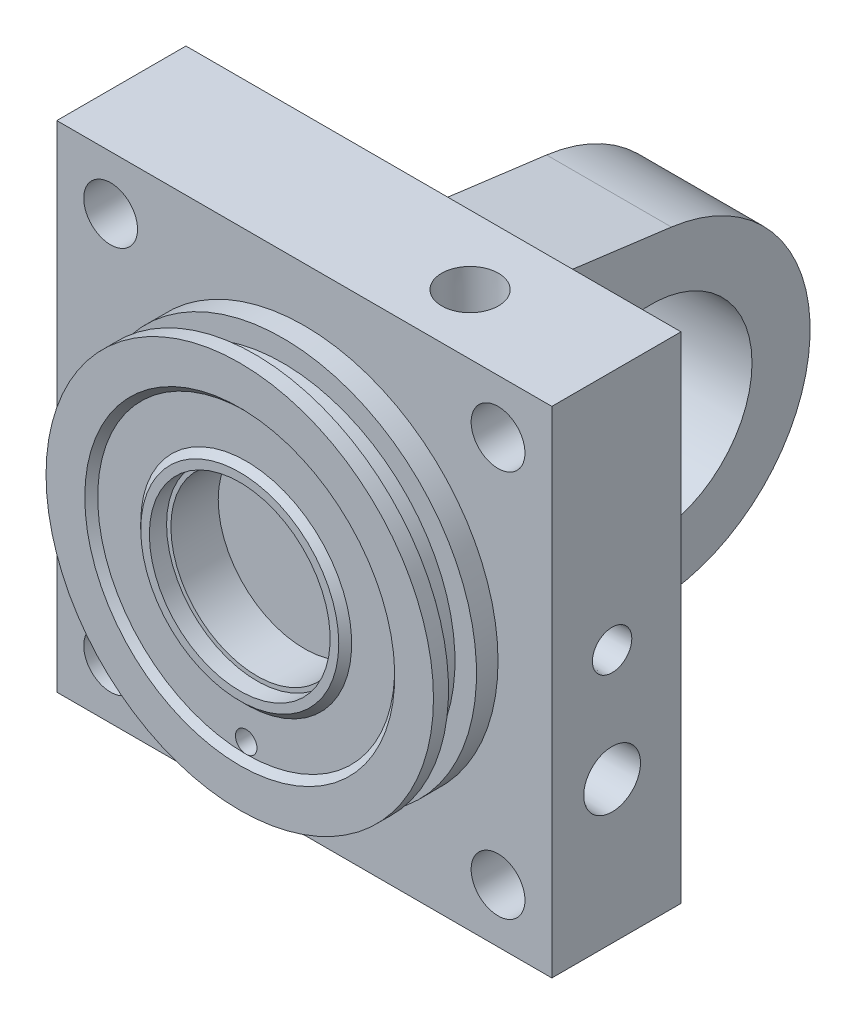
SolidWorks part; units mm, degrees
ref_plane "前视基准面" through (0, 0, 0) normal (0, 0, 1) x (1, 0, 0)
ref_plane "上视基准面" through (0, 0, 0) normal (0, 1, 0) x (1, 0, 0)
ref_plane "右视基准面" through (0, 0, 0) normal (1, 0, 0) x (0, 0, -1)
other "Configuration Table"
sketch "草图1" plane through (0, 0, 0) normal (0, 0, 1) x (1, 0, 0)
  line L1 (-57.5, -57.5) -> (57.5, -57.5)
  line L2 (-57.5, -57.5) -> (-57.5, 57.5)
  line L3 (-57.5, 57.5) -> (57.5, 57.5)
  line L4 (57.5, -57.5) -> (57.5, 57.5)
  line L5 (0, 57.5) -> (0, -57.5) construction
  line L6 (-57.5, 0) -> (57.5, 0) construction
  circle A0 centre (-45, 45) radius 6.25
  circle A1 centre (45, 45) radius 6.25
  circle A2 centre (45, -45) radius 6.25
  circle A3 centre (-45, -45) radius 6.25
  point P0 (0, 0)
  dimension "D3" = 12.5
  dimension "D12" = 12.5
  dimension "D6" = 12.5
  dimension "D7" = 12.5
  dimension "D8" = 12.5
  dimension "D1" = 115
  dimension "D2" = 115
  dimension "D4" = 45
  dimension "D5" = 12.5
  dimension "D9" = 12.5
  dimension "D10" = 90
  dimension "D11" = 12.5
extrude "凸台-拉伸1" add sketch "草图1" along normal blind 30
sketch "草图2" plane through (0, 0, 30) normal (0, 0, 1) x (1, 0, 0)
  circle A0 centre (0, 0) radius 45
  dimension "D1" = 90
extrude "凸台-拉伸2" add sketch "草图2" along normal blind 15
sketch "草图3" plane through (0, 0, 0) normal (1, 0, 0) x (0, 0, -1)
  line L0 (0, 0) -> (-45, 0) construction
  line L1 (-45, 45) -> (-45, -45) construction
  line L2 (-30, 20) -> (-41, 20)
  line L3 (-41, 20) -> (-41, 21)
  line L4 (-41, 21) -> (-45, 21)
  line L5 (-45, 21) -> (-45, 0)
  line L6 (-30, -57.5) -> (-30, 57.5) construction
  line L7 (-45, 23) -> (-43.5, 24.5)
  line L8 (-43.5, 24.5) -> (-43.5, 34.5)
  line L9 (-43.5, 34.5) -> (-45, 36)
  line L10 (-45, 36) -> (-45, 23)
  line L11 (-30, 45) -> (-45, 45) construction
  line L12 (-41.5, 45) -> (-35, 45)
  line L13 (-41.5, 45) -> (-41.5, 40)
  line L14 (-41.5, 40) -> (-35, 40)
  line L15 (-35, 45) -> (-35, 40)
  line L16 (-30, 20) -> (-30, 0)
  line L17 (-30, 45) -> (-30, -45) construction
  line L18 (-30, 0) -> (-45, 0)
  dimension "D1" = 21
  dimension "D2" = 4
  dimension "D3" = 20
  dimension "D4" = 23
  dimension "D5" = 1.5
  dimension "D6" = 36
  dimension "D7" = 40
  dimension "D8" = 3.5
  dimension "D9" = 6.5
  dimension "D10" = 45
  dimension "D11" = 45
revolve "切除-旋转1" cut sketch "草图3" angle 360 about L0
sketch "草图4" plane through (0, 0, 43.5) normal (0, 0, 1) x (1, 0, 0)
  circle A0 centre (0, -32) radius 2.5
  dimension "D1" = 5
  dimension "D2" = 32
extrude "切除-拉伸1" cut sketch "草图4" against normal blind 25
sketch "草图7" plane through (0, -57.5, 0) normal (0, -1, 0) x (-1, 0, 0)
  line L0 (-57.5, -30) -> (-57.5, 0) construction
  line L1 (57.5, 0) -> (-57.5, 0) construction
  point P0 (7.5, -16)
  dimension "D1" = 65
  dimension "D2" = 16
hole_wizard "1/4 NPT 螺纹孔1" positions "草图7" profile "草图6" size "1/4" standard "ANSI Inch"
sketch "草图6" plane through (-7.5, -57.5, 16) normal (1, 0, 0) x (0, 0, -1)
  line L0 (0, 0) -> (0, 35.3908)
  line L1 (5.5626, 32.0485) -> (0, 35.3908)
  line L2 (-5.5626, 32.0485) -> (0, 35.3908) construction
  line L3 (5.5626, 32.0485) -> (5.5626, 25)
  line L4 (5.5626, 25) -> (5.9437, 25)
  line L5 (5.9437, 25) -> (6.6922, 0)
  line L6 (-5.9437, 25) -> (-6.6922, 0) construction
  line L7 (6.6922, 0) -> (0, 0)
  line L8 (0, -6.35) -> (0, 107.95) construction
  line L11 (-5.5626, 25) -> (-5.9437, 25) construction
  dimension "螺纹孔钻头直径" = 11.1252
  dimension "螺纹孔钻头深度" = 32.0485
  dimension "螺纹直径" = 13.3844
  dimension "螺纹角度" = 3.43
  dimension "螺纹深度" = 25
  dimension "导头角度" = 118
cosmetic thread "孔螺纹线1" parameters "D1"=25, "D2"=14.6125
sketch "草图10" plane through (57.5, 0, 0) normal (1, 0, 0) x (0, 0, -1)
  line L0 (-30, 57.5) -> (0, 57.5) construction
  line L1 (0, -57.5) -> (0, 57.5) construction
  point P0 (-16, -24.5)
  dimension "D1" = 82
  dimension "D2" = 16
hole_wizard "1/4 Rc 螺纹孔1" positions "草图10" profile "草图9" size "1/4" standard "GB"
sketch "草图9" plane through (57.5, -24.5, 16) normal (0, 1, 0) x (0, 0, -1)
  line L0 (0, 0) -> (0, 34.8996)
  line L1 (5.35, 31.685) -> (0, 34.8996)
  line L2 (-5.35, 31.685) -> (0, 34.8996) construction
  line L3 (5.35, 31.685) -> (5.35, 25)
  line L4 (5.35, 25) -> (5.8106, 25)
  line L5 (5.8106, 25) -> (6.591, 0)
  line L6 (-5.8106, 25) -> (-6.591, 0) construction
  line L7 (6.591, 0) -> (0, 0)
  line L8 (0, -6.35) -> (0, 107.95) construction
  line L11 (-5.35, 25) -> (-5.8106, 25) construction
  dimension "螺纹孔钻头直径" = 10.7
  dimension "螺纹孔钻头深度" = 31.685
  dimension "螺纹直径" = 13.1821
  dimension "螺纹角度" = 3.576
  dimension "螺纹深度" = 25
  dimension "导头角度" = 118
cosmetic thread "孔螺纹线2" parameters "D1"=25, "D2"=14.0446
sketch "草图13" plane through (57.5, 0, 0) normal (1, 0, 0) x (0, 0, -1)
  line L0 (-30, 57.5) -> (0, 57.5) construction
  line L1 (0, -57.5) -> (0, 57.5) construction
  point P0 (-16, 1.5)
  dimension "D1" = 56
  dimension "D2" = 16
hole_wizard "1/8 Rc 螺纹孔1" positions "草图13" profile "草图12" size "1/8" standard "GB"
sketch "草图12" plane through (57.5, 1.5, 16) normal (0, 1, 0) x (0, 0, -1)
  line L0 (0, 0) -> (0, 14.3134)
  line L1 (3.95, 11.94) -> (0, 14.3134)
  line L2 (-3.95, 11.94) -> (0, 14.3134) construction
  line L3 (3.95, 11.94) -> (3.95, 7.4)
  line L4 (3.95, 7.4) -> (4.3425, 7.4)
  line L5 (4.3425, 7.4) -> (4.5735, 0)
  line L6 (-4.3425, 7.4) -> (-4.5735, 0) construction
  line L7 (4.5735, 0) -> (0, 0)
  line L8 (0, -6.35) -> (0, 107.95) construction
  line L11 (-3.95, 7.4) -> (-4.3425, 7.4) construction
  dimension "螺纹孔钻头直径" = 7.9
  dimension "螺纹孔钻头深度" = 11.94
  dimension "螺纹直径" = 9.147
  dimension "螺纹角度" = 3.576
  dimension "螺纹深度" = 7.4
  dimension "导头角度" = 118
cosmetic thread "孔螺纹线3" parameters "D1"=7.4, "D2"=11.7267
sketch "草图16" plane through (0, 57.5, 0) normal (0, 1, 0) x (1, 0, 0)
  line L0 (-57.5, -30) -> (-57.5, 0) construction
  line L1 (57.5, 0) -> (-57.5, 0) construction
  point P0 (24.5, -16)
  dimension "D1" = 82
  dimension "D2" = 16
hole_wizard "1/4 Rc 螺纹孔2" positions "草图16" profile "草图15" size "1/4" standard "GB"
sketch "草图15" plane through (24.5, 57.5, 16) normal (1, 0, 0) x (0, 0, 1)
  line L0 (0, 0) -> (0, 34.8996)
  line L1 (5.35, 31.685) -> (0, 34.8996)
  line L2 (-5.35, 31.685) -> (0, 34.8996) construction
  line L3 (5.35, 31.685) -> (5.35, 25)
  line L4 (5.35, 25) -> (5.8106, 25)
  line L5 (5.8106, 25) -> (6.591, 0)
  line L6 (-5.8106, 25) -> (-6.591, 0) construction
  line L7 (6.591, 0) -> (0, 0)
  line L8 (0, -6.35) -> (0, 107.95) construction
  line L11 (-5.35, 25) -> (-5.8106, 25) construction
  dimension "螺纹孔钻头直径" = 10.7
  dimension "螺纹孔钻头深度" = 31.685
  dimension "螺纹直径" = 13.1821
  dimension "螺纹角度" = 3.576
  dimension "螺纹深度" = 25
  dimension "导头角度" = 118
cosmetic thread "孔螺纹线4" parameters "D1"=25, "D2"=14.0446
sketch "草图17" plane through (0, 57.5, 0) normal (0, 1, 0) x (1, 0, 0)
  circle A0 centre (24.5, -16) radius 3
  dimension "D1" = 6
extrude "切除-拉伸2" cut sketch "草图17" against normal blind 43
sketch "草图18" plane through (57.5, 0, 0) normal (1, 0, 0) x (0, 0, -1)
  circle A0 centre (-16, 1.5) radius 3
  circle A1 centre (-16, -24.5) radius 3
  dimension "D1" = 6
  dimension "D2" = 6
extrude "切除-拉伸3" cut sketch "草图18" against normal blind 69
sketch "草图19" plane through (0, -57.5, 0) normal (0, -1, 0) x (1, 0, 0)
  circle A0 centre (-7.5, 16) radius 3
  dimension "D1" = 6
extrude "切除-拉伸4" cut sketch "草图19" against normal blind 82
sketch "草图20" plane through (0, 0, 0) normal (1, 0, 0) x (0, 0, -1)
  line L0 (0, 0) -> (95.8913, 0) construction
  line L1 (0, 42) -> (0, -42)
  line L2 (0, -57.5) -> (0, 57.5) construction
  line L3 (0, -42) -> (40.7775, -36.6903)
  line L4 (-45, 45) -> (-45, -45) construction
  line L5 (0, 42) -> (40.7775, 36.6903)
  arc A0 (40.7775, -36.6903) -> (40.7775, 36.6903) centre (36, 0) ccw
  circle A1 centre (36, 0) radius 23.5
  dimension "D1" = 37
  dimension "D4" = 47
  dimension "D2" = 42
  dimension "D3" = 81
extrude "凸台-拉伸3" add sketch "草图20" along normal mid plane 29
equation "\"69、\"=43"
